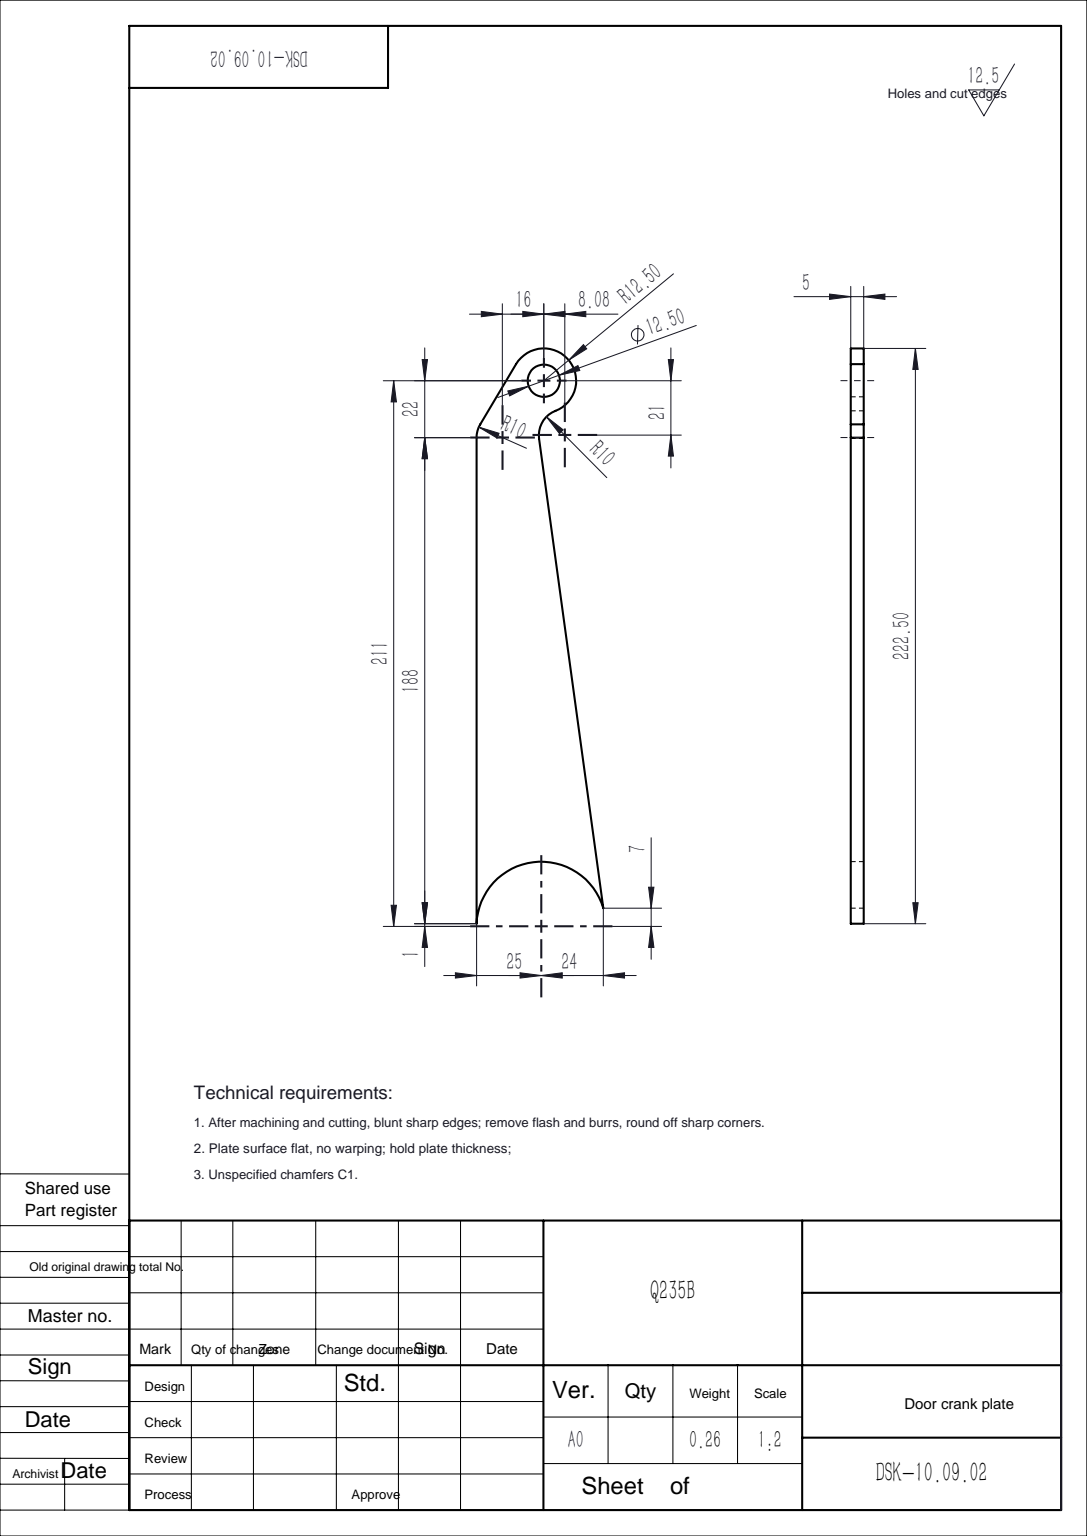
from build123d import *

# Parameters (mm, degrees)
SKETCH1_R           = 12.5
SKETCH1_R_2         = 6.25
BOSS_EXTRUDE1_DEPTH = 5


with BuildPart() as part:
    # Sketch1 → Boss-Extrude1 (new body)
    # profile 1 of 2: a face of its own
    with BuildSketch(Plane.XY):
        with BuildLine():
            Line((-24.979991994, 189), (-24.979991994, 1))
            ThreePointArc((-24.979991994, 1), (-3.039752634, 24.814509947), (24, 7))
            Line((24, 7), (-0.810252343, 188.64671282))
            ThreePointArc((-0.810252343, 188.64671282), (0.4895755, 195.089129783), (5.507645346, 199.333333333))
            ThreePointArc((5.507645346, 199.333333333), (-8.535525821, 202.941354129), (-9.722087316, 217.391978417))
            Line((-9.722087316, 217.391978417), (-23.573668252, 194.113582733))
            ThreePointArc((-23.573668252, 194.113582733), (-24.622003262, 191.651719953), (-24.979991994, 189))
        make_face()
    # profile 2 of 2: a face of its own
    with BuildSketch(Plane.XY):
        with Locations((1.020008006, 211)):
            Circle(SKETCH1_R)
        with Locations((1.020008006, 211)):
            Circle(SKETCH1_R_2, mode=Mode.SUBTRACT)
    extrude(amount=BOSS_EXTRUDE1_DEPTH)


solid = part.part
